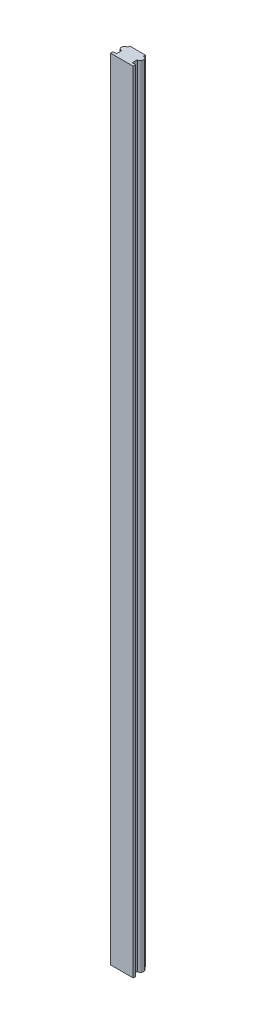
SolidWorks part; units mm, degrees
ref_plane "前视基准面" through (0, 0, 0) normal (0, 0, 1) x (1, 0, 0)
ref_plane "上视基准面" through (0, 0, 0) normal (0, 1, 0) x (1, 0, 0)
ref_plane "右视基准面" through (0, 0, 0) normal (1, 0, 0) x (0, 0, -1)
sketch "草图1" plane through (0, 0, 0) normal (0, 1, 0) x (1, 0, 0)
  line L0 (0, 0) -> (0, 11.3364) construction
  line L1 (-12.5, 5) -> (-12.5, 8)
  line L2 (-12.5, 8) -> (12.5, 8)
  line L3 (12.5, 8) -> (12.5, 5)
  line L4 (-12.5, -5) -> (-12.5, -13)
  line L5 (-12.5, -13) -> (-18, -13)
  line L6 (-18, -13) -> (-18, -17)
  line L7 (-18, -17) -> (18, -17)
  line L8 (18, -17) -> (18, -13)
  line L9 (18, -13) -> (12.5, -13)
  line L10 (12.5, -13) -> (12.5, -5)
  arc A0 (-12.5, 5) -> (-12.5, -5) centre (-12.5, 0) ccw
  arc A1 (12.5, -5) -> (12.5, 5) centre (12.5, 0) ccw
  dimension "D1" = 10
  dimension "D3" = 36
  dimension "D2" = 25
  dimension "D4" = 17
  dimension "D5" = 25
  dimension "D6" = 4
extrude "凸台-拉伸1" add sketch "草图1" along normal blind 1252
ref_plane "基准面1" through (0, 0, 0) normal (0, 0, 1) x (1, 0, 0)
